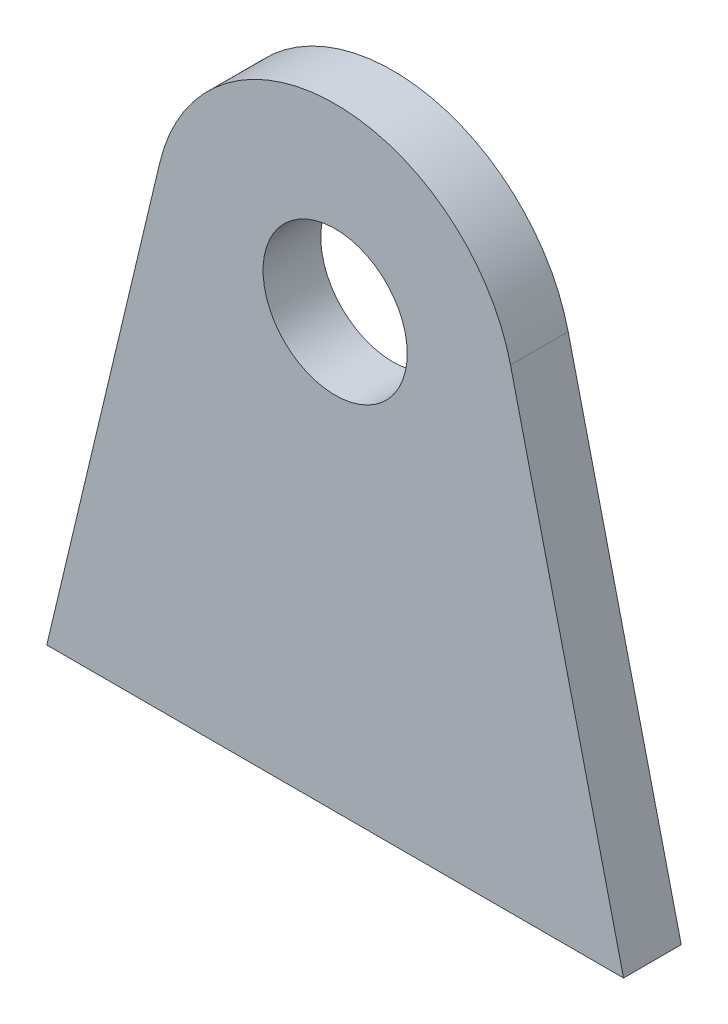
SolidWorks part; units mm, degrees
ref_plane "前视基准面" through (0, 0, 0) normal (0, 0, 1) x (1, 0, 0)
ref_plane "上视基准面" through (0, 0, 0) normal (0, 1, 0) x (1, 0, 0)
ref_plane "右视基准面" through (0, 0, 0) normal (1, 0, 0) x (0, 0, -1)
sketch "草图1" plane through (0, 0, 0) normal (0, 0, 1) x (1, 0, 0)
  line L0 (0, 0) -> (80, 0)
  line L3 (0, 0) -> (15.6811, 65.7959)
  line L4 (80, 0) -> (64.3189, 65.7959)
  arc A0 (64.3189, 65.7959) -> (15.6811, 65.7959) centre (40, 60) ccw
  circle A1 centre (40, 60) radius 10
extrude "凸台-拉伸1" add sketch "草图1" along normal blind 8
